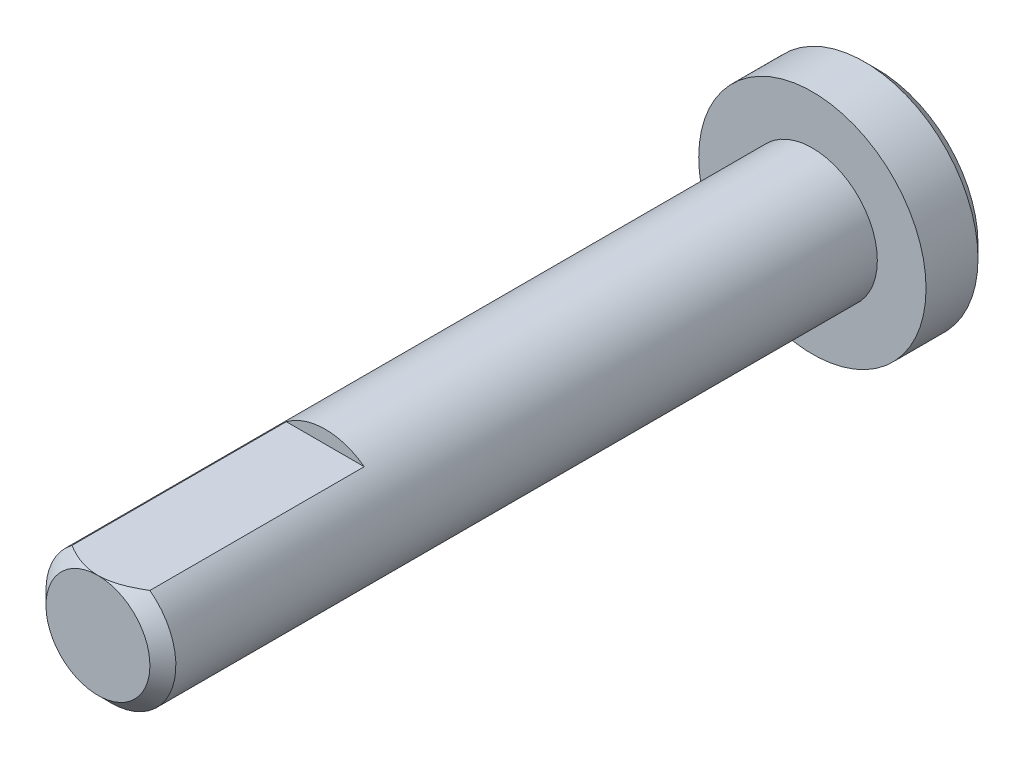
from build123d import *

# Parameters (mm, degrees)
SKETCH1_R           = 1.75
BOSS_EXTRUDE1_DEPTH = 1
SKETCH2_R           = 1
BOSS_EXTRUDE2_DEPTH = 11
CHAMFER1_SIZE       = 0.2
CUT_EXTRUDE1_START  = -3.5
CUT_EXTRUDE1_DEPTH  = 3.5


with BuildPart() as part:
    # Sketch1 → Boss-Extrude1 (new body)
    with BuildSketch(Plane.XY):
        Circle(SKETCH1_R)
    extrude(amount=BOSS_EXTRUDE1_DEPTH)

    # Sketch2 → Boss-Extrude2 (add)
    with BuildSketch(Plane.XY.offset(1)):
        Circle(SKETCH2_R)
    extrude(amount=BOSS_EXTRUDE2_DEPTH)

    # Chamfer1
    chamfer1_edges = [part.edges().sort_by_distance(p)[0] for p in [
        (-1.75, 0, 0),
        (-1, 0, 12),
    ]]
    chamfer(chamfer1_edges, length=CHAMFER1_SIZE)

    # Sketch3 → Cut-Extrude1 (cut)
    with BuildSketch(Plane.XY.offset(12).offset(CUT_EXTRUDE1_START)):
        with BuildLine():
            Line((-0.6, 0.8), (0.6, 0.8))
            ThreePointArc((0.6, 0.8), (0, 1), (-0.6, 0.8))
        make_face()
    extrude(amount=CUT_EXTRUDE1_DEPTH, mode=Mode.SUBTRACT)


solid = part.part
